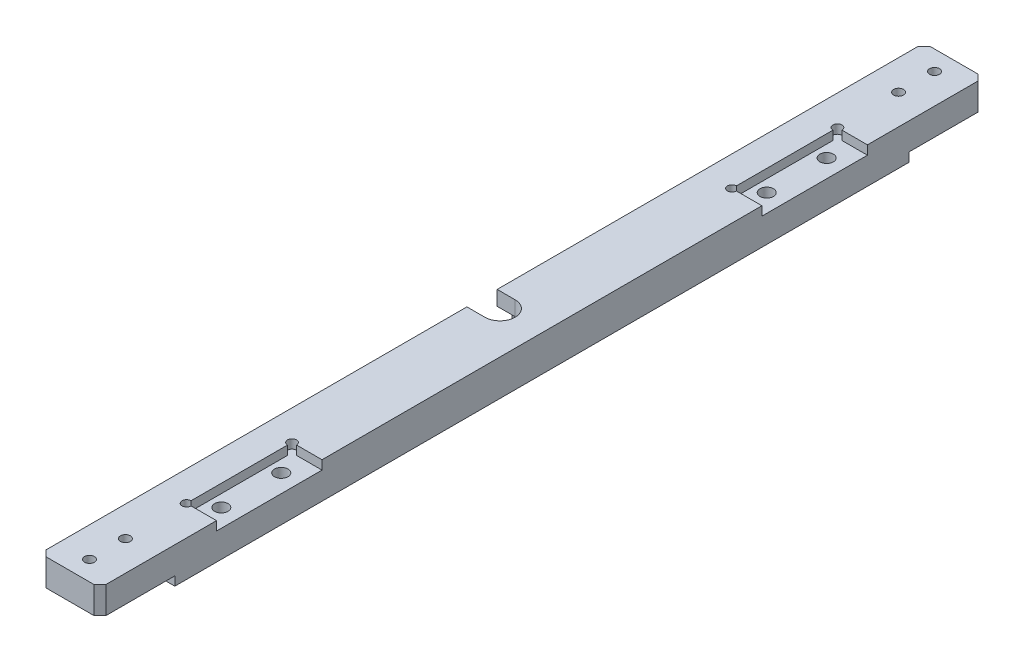
from build123d import *

# Parameters (mm, degrees)
SKETCH1_W                                            = 295
SKETCH1_H                                            = 12
BOSS_EXTRUDE1_DEPTH                                  = 20
CUT_EXTRUDE1_DEPTH                                   = 150.33268229
CUT_EXTRUDE2_DEPTH                                   = 7.1
SKETCH4_W                                            = 20
SKETCH4_H                                            = 25
CUT_EXTRUDE3_DEPTH                                   = 3
SKETCH5_W                                            = 10
SKETCH5_H                                            = 35.2
CUT_EXTRUDE4_DEPTH                                   = 3
SKETCH7_R                                            = 1.5
CUT_EXTRUDE6_DEPTH                                   = 3
M4_TAPPED_HOLE2_D                                    = 3.3
M4_TAPPED_HOLE2_DEPTH                                = 10.1
M4_TAPPED_HOLE2_TIP                                  = 0.991420021
M4_TAPPED_HOLE1_D                                    = 3.3
M4_TAPPED_HOLE1_DEPTH                                = 10.1
M4_TAPPED_HOLE1_TIP                                  = 0.991420021
CBORE_FOR_M4_HEXAGON_SOCKET_HEAD_CAP_SCR_D           = 4.5
CBORE_FOR_M4_HEXAGON_SOCKET_HEAD_CAP_SCR_CBORE_D     = 8
CBORE_FOR_M4_HEXAGON_SOCKET_HEAD_CAP_SCR_CBORE_DEPTH = 4.6
CHAMFER1_SIZE                                        = 2


with BuildPart() as part:
    # Sketch1 → Boss-Extrude1 (new body)
    with BuildSketch(Plane(origin=(0, 0, 0), x_dir=(0, 0, -1), z_dir=(1, 0, 0))):
        Rectangle(SKETCH1_W, SKETCH1_H)
    extrude(amount=BOSS_EXTRUDE1_DEPTH)

    # Sketch2 → Cut-Extrude1 (cut, through all)
    with BuildSketch(Plane.XZ.offset(6)):
        with BuildLine():
            Line((0, 5.05), (6, 5.05))
            ThreePointArc((6, 5.05), (11.05, 0), (6, -5.05))
            Line((6, -5.05), (0, -5.05))
            ThreePointArc((0, -5.05), (-5.05, 0), (0, 5.05))
        make_face()
    extrude(amount=-CUT_EXTRUDE1_DEPTH, mode=Mode.SUBTRACT)

    # Sketch3 → Cut-Extrude2 (cut)
    with BuildSketch(Plane.XZ.offset(6)):
        with BuildLine():
            Line((0, 10), (6, 10))
            ThreePointArc((6, 10), (16, 0), (6, -10))
            Line((6, -10), (0, -10))
            ThreePointArc((0, -10), (-10, 0), (0, 10))
        make_face()
    extrude(amount=-CUT_EXTRUDE2_DEPTH, mode=Mode.SUBTRACT)

    # Sketch4 → Cut-Extrude3 (cut)
    with BuildSketch(Plane(origin=(0, -6, 0), x_dir=(1, 0, 0), z_dir=(0, 1, 0))):
        with Locations((10, -135)):
            Rectangle(SKETCH4_W, SKETCH4_H)
        with Locations((10, 135)):
            Rectangle(SKETCH4_W, SKETCH4_H)
    extrude(amount=CUT_EXTRUDE3_DEPTH, mode=Mode.SUBTRACT)

    # Sketch5 → Cut-Extrude4 (cut)
    with BuildSketch(Plane(origin=(0, 6, 0), x_dir=(1, 0, 0), z_dir=(0, 1, 0))):
        with Locations((15, 91)):
            Rectangle(SKETCH5_W, SKETCH5_H)
        with Locations((15, -91)):
            Rectangle(SKETCH5_W, SKETCH5_H)
    extrude(amount=-CUT_EXTRUDE4_DEPTH, mode=Mode.SUBTRACT)

    # Sketch7 → Cut-Extrude6 (cut)
    with BuildSketch(Plane(origin=(0, 6, 0), x_dir=(1, 0, 0), z_dir=(0, 1, 0))):
        with Locations((10, 108.6)):
            Circle(SKETCH7_R)
        with Locations((10, 73.4)):
            Circle(SKETCH7_R)
        with Locations((10, -73.4)):
            Circle(SKETCH7_R)
        with Locations((10, -108.6)):
            Circle(SKETCH7_R)
    extrude(amount=-CUT_EXTRUDE6_DEPTH, mode=Mode.SUBTRACT)

    # M4 Tapped Hole2
    with Locations(Plane(origin=(0, -3, 0), x_dir=(-1, 0, 0), z_dir=(0, -1, 0))):
        with Locations((-10, -141), (-10, -129)):
            Hole(M4_TAPPED_HOLE2_D / 2, depth=M4_TAPPED_HOLE2_DEPTH)
            with Locations((0, 0, -(M4_TAPPED_HOLE2_DEPTH + M4_TAPPED_HOLE2_TIP / 2))):  # 118° drill point
                Cone(0, M4_TAPPED_HOLE2_D / 2, M4_TAPPED_HOLE2_TIP, mode=Mode.SUBTRACT)

    # M4 Tapped Hole1
    with Locations(Plane(origin=(0, -3, 0), x_dir=(-1, 0, 0), z_dir=(0, -1, 0))):
        with Locations((-10, 141), (-10, 129)):
            Hole(M4_TAPPED_HOLE1_D / 2, depth=M4_TAPPED_HOLE1_DEPTH)
            with Locations((0, 0, -(M4_TAPPED_HOLE1_DEPTH + M4_TAPPED_HOLE1_TIP / 2))):  # 118° drill point
                Cone(0, M4_TAPPED_HOLE1_D / 2, M4_TAPPED_HOLE1_TIP, mode=Mode.SUBTRACT)

    # CBORE for M4 Hexagon socket head cap screws1 (through all)
    with Locations(Plane(origin=(0, -6, 0), x_dir=(-1, 0, 0), z_dir=(0, -1, 0))):
        with Locations((-14, 101), (-14, 81), (-14, -81), (-14, -101)):
            CounterBoreHole(CBORE_FOR_M4_HEXAGON_SOCKET_HEAD_CAP_SCR_D / 2, CBORE_FOR_M4_HEXAGON_SOCKET_HEAD_CAP_SCR_CBORE_D / 2, CBORE_FOR_M4_HEXAGON_SOCKET_HEAD_CAP_SCR_CBORE_DEPTH)

    # Chamfer1
    chamfer1_edges = [part.edges().sort_by_distance(p)[0] for p in [
        (20, 1.5, 147.5),
        (0, 1.5, 147.5),
        (0, 1.5, -147.5),
        (20, 1.5, -147.5),
    ]]
    chamfer(chamfer1_edges, length=CHAMFER1_SIZE)


solid = part.part
